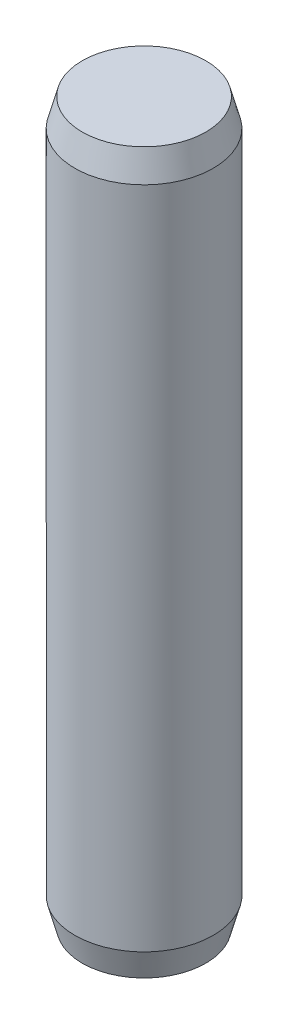
from build123d import *

# Parameters (mm, degrees)
SKETCH1_R           = 2.5
BOSS_EXTRUDE1_DEPTH = 13
CHAMFER1_SIZE       = 1
CHAMFER1_SIZE2      = 0.267949192
CHAMFER3_SIZE       = 0.27
CHAMFER3_SIZE2      = 1.007653718


with BuildPart() as part:
    # Sketch1 → Boss-Extrude1 (new, symmetric)
    with BuildSketch(Plane(origin=(0, 0, 0), x_dir=(1, 0, 0), z_dir=(0, 1, 0))):
        with Locations(Location((0, 0, 0), (0, 0, 90))):
            Circle(SKETCH1_R)
    extrude(amount=BOSS_EXTRUDE1_DEPTH, both=True)

    # Chamfer1
    chamfer1_edges = [part.edges().sort_by_distance(p)[0] for p in [
        (0, 13, 2.5),
    ]]
    chamfer1_side = [part.faces().sort_by_distance(p)[0] for p in [
        (0, 0, 2.5),
    ]]
    chamfer(chamfer1_edges, length=CHAMFER1_SIZE, length2=CHAMFER1_SIZE2, reference=chamfer1_side[0])

    # Chamfer3
    chamfer3_edges = [part.edges().sort_by_distance(p)[0] for p in [
        (0, -13, 2.5),
    ]]
    chamfer3_side = [part.faces().sort_by_distance(p)[0] for p in [
        (0, -13, 0),
    ]]
    chamfer(chamfer3_edges, length=CHAMFER3_SIZE, length2=CHAMFER3_SIZE2, reference=chamfer3_side[0])


solid = part.part
